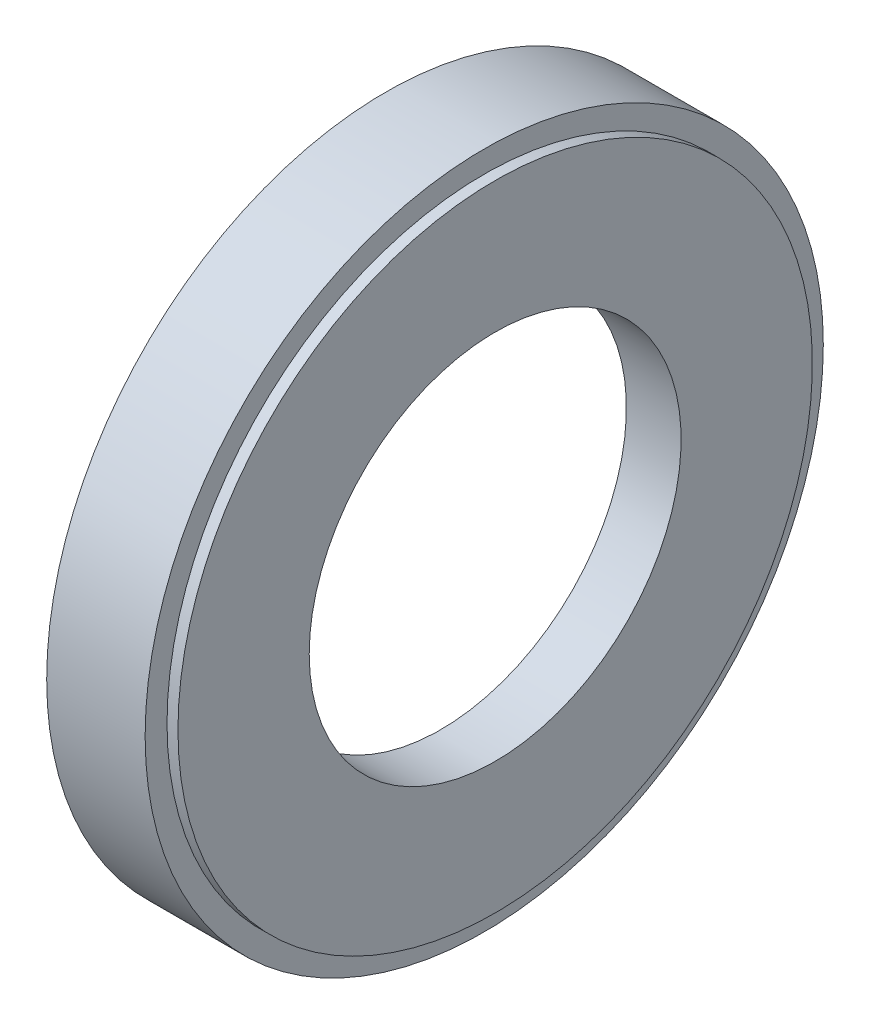
SolidWorks part; units mm, degrees
ref_plane "前视基准面" through (0, 0, 0) normal (0, 0, 1) x (1, 0, 0)
ref_plane "上视基准面" through (0, 0, 0) normal (0, 1, 0) x (1, 0, 0)
ref_plane "右视基准面" through (0, 0, 0) normal (1, 0, 0) x (0, 0, -1)
sketch "草图1" plane through (0, 0, 0) normal (0, 0, 1) x (1, 0, 0)
  line L0 (0, 0) -> (24.1292, 0) construction
  line L1 (-1.6467, 17) -> (3.3533, 17)
  line L2 (3.3533, 17) -> (3.3533, 29)
  line L3 (3.3533, 29) -> (2.3533, 29)
  line L4 (2.3533, 29) -> (2.3533, 31)
  line L5 (2.3533, 31) -> (-6.6467, 31)
  line L6 (-6.6467, 31) -> (-6.6467, 29)
  line L7 (-6.6467, 29) -> (-1.6467, 29)
  line L8 (-1.6467, 29) -> (-1.6467, 17)
  dimension "D1" = 9
  dimension "D2" = 1
  dimension "D3" = 5
  dimension "D4" = 5
  dimension "D5" = 12
  dimension "D6" = 2
  dimension "D7" = 2
  dimension "D8" = 17
revolve "旋转1" add sketch "草图1" angle 360 about L0
